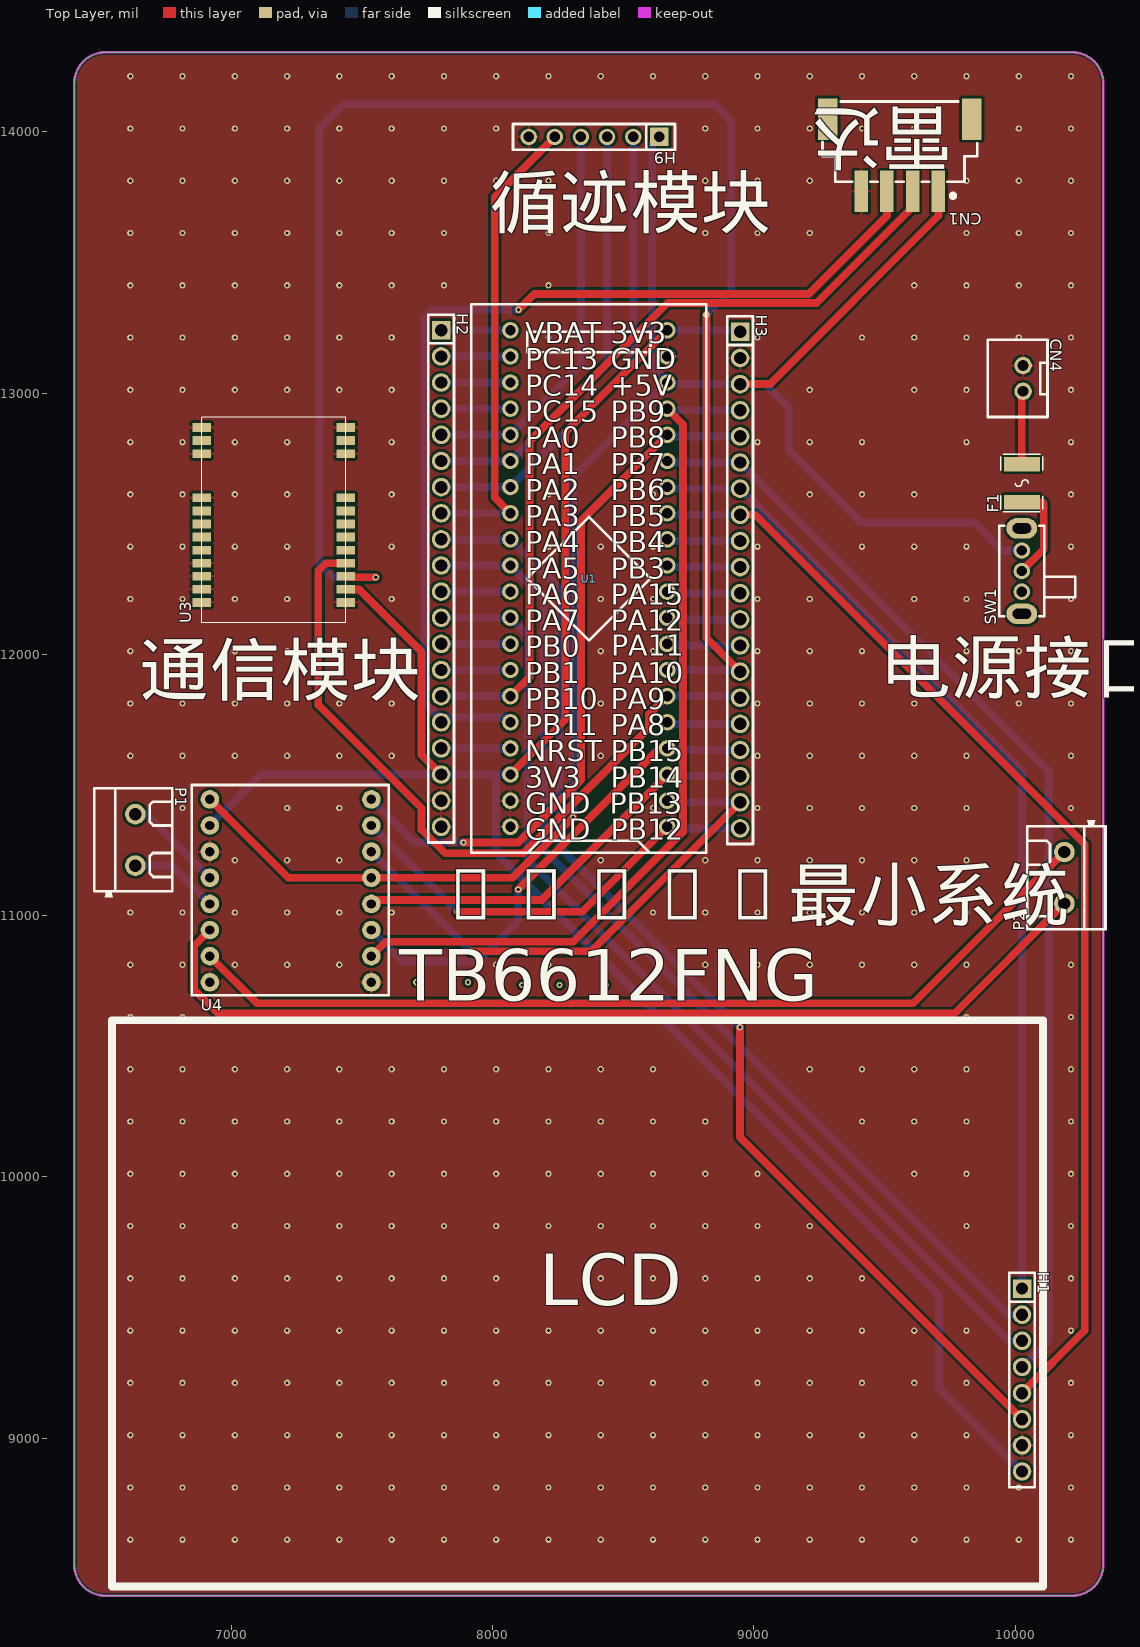
[diagram p0: Top Layer view]
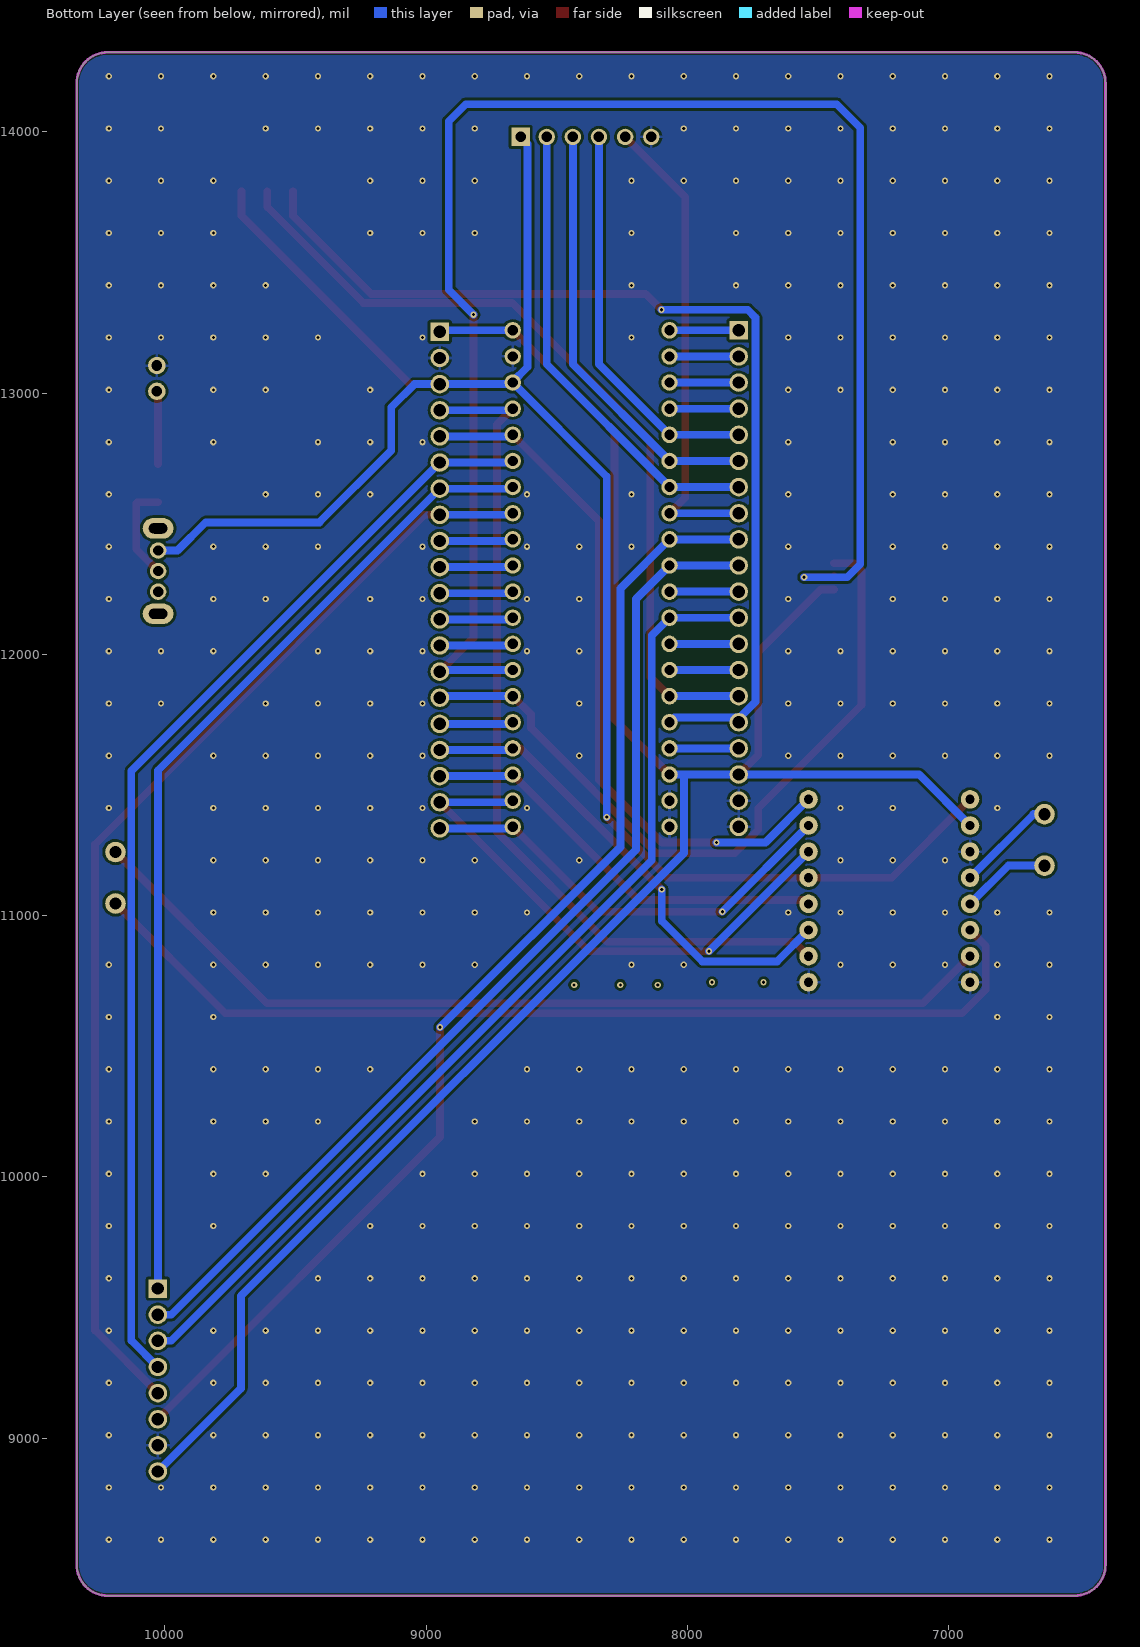
[diagram p1: Bottom Layer view, seen from below]
# Altium PCB MISC52128.pcbdoc
Units mil, origin at the board's own origin, x right, y up, seen from the top; angles counter-clockwise.
Board outline 3937.01 x 5905.51 mil, 2 copper layers (Top Layer, Bottom Layer), stack 62.206 mil thick; 13 components, 43 nets, 153 pads, 421 vias.

## Layer stack, top to bottom
Top Solder Mask Layer: solder mask 0.394, Dk 3.3
Top Layer: signal copper 1.379
Dielectric1: surface 59.449, FR4, Dk 4.5
Bottom Layer: signal copper 1.378
Bottom Solder Mask Layer: solder mask 0.394, Dk 3.3

## Board outline
6517.91,14303.5 ccw(c6517.91,14185.39) 6399.8,14185.39 6399.8,8516.1 ccw(c6517.91,8516.1) 6517.91,8397.99 10218.7,8397.99 ccw(c10218.7,8516.1) 10336.81,8516.1 10336.81,14185.39 ccw(c10218.7,14185.39) 10218.7,14303.5 6517.91,14303.5

## Design rules (kind name [scope] priority, off if disabled: settings)
BoardOutlineClearance copperThickness2oz_1 [All] p2 off: genericclearance=7.99 ignorepadtopadclearanceinfootprint=FALSE except(0: Arc-SplitContinuation Track-SplitContinuation SMDPad-SplitContinuation THPad-SplitContinuation Via-SplitContinuation Fill-SplitContinuation Region-SplitContinuation Poly-SplitContinuation Text-SplitContinuation Hole-SplitContinuation; 5.98: Arc-CutoutEdge Track-CutoutEdge SMDPad-CutoutEdge THPad-CutoutEdge Via-CutoutEdge Text-CutoutEdge; 6.9: Hole-OutlineEdge Hole-CutoutEdge; 10: Poly-OutlineEdge Poly-CutoutEdge; 11.81: Arc-OutlineEdge Track-OutlineEdge SMDPad-OutlineEdge THPad-OutlineEdge Via-OutlineEdge Fill-OutlineEdge Region-OutlineEdge Text-OutlineEdge Fill-CutoutEdge Region-CutoutEdge)
BoardOutlineClearance Plane_innerPlane_1 [All] p4 off: genericclearance=4.02 ignorepadtopadclearanceinfootprint=FALSE except(0: Arc-SplitContinuation Track-SplitContinuation SMDPad-SplitContinuation THPad-SplitContinuation Via-SplitContinuation Fill-SplitContinuation Region-SplitContinuation Poly-SplitContinuation Text-SplitContinuation Hole-SplitContinuation; 5.98: Arc-CutoutEdge Track-CutoutEdge SMDPad-CutoutEdge THPad-CutoutEdge Via-CutoutEdge Text-CutoutEdge; 6.9: Hole-OutlineEdge Hole-CutoutEdge; 10: Poly-OutlineEdge Poly-CutoutEdge; 11.81: Arc-OutlineEdge Track-OutlineEdge SMDPad-OutlineEdge THPad-OutlineEdge Via-OutlineEdge Fill-OutlineEdge Region-OutlineEdge Text-OutlineEdge Fill-CutoutEdge Region-CutoutEdge)
BoardOutlineClearance Copper_copperRegion_1 [All] p6 off: genericclearance=4.02 ignorepadtopadclearanceinfootprint=FALSE except(0: Arc-SplitContinuation Track-SplitContinuation SMDPad-SplitContinuation THPad-SplitContinuation Via-SplitContinuation Fill-SplitContinuation Region-SplitContinuation Poly-SplitContinuation Text-SplitContinuation Hole-SplitContinuation; 5.98: Arc-CutoutEdge Track-CutoutEdge SMDPad-CutoutEdge THPad-CutoutEdge Via-CutoutEdge Text-CutoutEdge; 6.9: Hole-OutlineEdge Hole-CutoutEdge; 10: Poly-OutlineEdge Poly-CutoutEdge; 11.81: Arc-OutlineEdge Track-OutlineEdge SMDPad-OutlineEdge THPad-OutlineEdge Via-OutlineEdge Fill-OutlineEdge Region-OutlineEdge Text-OutlineEdge Fill-CutoutEdge Region-CutoutEdge)
BoardOutlineClearance Copper_copperRegion_copperThickness1oz_1 [All] p8 off: genericclearance=4.02 ignorepadtopadclearanceinfootprint=FALSE except(0: Arc-SplitContinuation Track-SplitContinuation SMDPad-SplitContinuation THPad-SplitContinuation Via-SplitContinuation Fill-SplitContinuation Region-SplitContinuation Poly-SplitContinuation Text-SplitContinuation Hole-SplitContinuation; 5.98: Arc-CutoutEdge Track-CutoutEdge SMDPad-CutoutEdge THPad-CutoutEdge Via-CutoutEdge Text-CutoutEdge; 6.9: Hole-OutlineEdge Hole-CutoutEdge; 10: Poly-OutlineEdge Poly-CutoutEdge; 11.81: Arc-OutlineEdge Track-OutlineEdge SMDPad-OutlineEdge THPad-OutlineEdge Via-OutlineEdge Fill-OutlineEdge Region-OutlineEdge Text-OutlineEdge Fill-CutoutEdge Region-CutoutEdge)
BoardOutlineClearance Copper_copperRegion_Copper_copperRegion_1 [All] p10 off: genericclearance=4.02 ignorepadtopadclearanceinfootprint=FALSE except(0: Arc-SplitContinuation Track-SplitContinuation SMDPad-SplitContinuation THPad-SplitContinuation Via-SplitContinuation Fill-SplitContinuation Region-SplitContinuation Poly-SplitContinuation Text-SplitContinuation Hole-SplitContinuation; 5.98: Arc-CutoutEdge Track-CutoutEdge SMDPad-CutoutEdge THPad-CutoutEdge Via-CutoutEdge Text-CutoutEdge; 6.9: Hole-OutlineEdge Hole-CutoutEdge; 10: Poly-OutlineEdge Poly-CutoutEdge; 11.81: Arc-OutlineEdge Track-OutlineEdge SMDPad-OutlineEdge THPad-OutlineEdge Via-OutlineEdge Fill-OutlineEdge Region-OutlineEdge Text-OutlineEdge Fill-CutoutEdge Region-CutoutEdge)
BoardOutlineClearance copperThickness1oz_1 [All] p12: genericclearance=4.02 ignorepadtopadclearanceinfootprint=FALSE except(0: Arc-SplitContinuation Track-SplitContinuation SMDPad-SplitContinuation THPad-SplitContinuation Via-SplitContinuation Fill-SplitContinuation Region-SplitContinuation Poly-SplitContinuation Text-SplitContinuation Hole-SplitContinuation; 5.98: Arc-CutoutEdge Track-CutoutEdge SMDPad-CutoutEdge THPad-CutoutEdge Via-CutoutEdge Text-CutoutEdge; 6.9: Hole-OutlineEdge Hole-CutoutEdge; 10: Poly-OutlineEdge Poly-CutoutEdge; 11.81: Arc-OutlineEdge Track-OutlineEdge SMDPad-OutlineEdge THPad-OutlineEdge Via-OutlineEdge Fill-OutlineEdge Region-OutlineEdge Text-OutlineEdge Fill-CutoutEdge Region-CutoutEdge)
Clearance copperThickness2oz [All] p1 off: gap=7.99 ignorepadtopadclearanceinfootprint=FALSE except(5.98: SMDPad-Track SMDPad-SMDPad THPad-Track SMDPad-THPad THPad-THPad Track-Via SMDPad-Via THPad-Via Via-Via Fill-SMDPad Region-SMDPad Fill-THPad Region-THPad Fill-Via Region-Via Fill-Fill Fill-Region Region-Region Arc-Track Arc-SMDPad Arc-THPad Arc-Via Fill-Arc Region-Arc Arc-Arc Text-Track SMDPad-Text Text-THPad Text-Via Fill-Text Region-Text Arc-Text Text-Text; 6.9: Hole-Track Hole-SMDPad Hole-THPad Hole-Via Fill-Hole Region-Hole Hole-Arc Hole-Text; 10: Poly-Track Poly-SMDPad Poly-THPad Poly-Via Poly-Fill Poly-Region Poly-Poly Poly-Arc Poly-Text Poly-Hole; 11.81: Fill-Track Region-Track)
Clearance Plane_innerPlane [All] p3 off: gap=4.02 ignorepadtopadclearanceinfootprint=FALSE except(5.98: SMDPad-Track SMDPad-SMDPad THPad-Track SMDPad-THPad THPad-THPad Track-Via SMDPad-Via THPad-Via Via-Via Fill-SMDPad Region-SMDPad Fill-THPad Region-THPad Fill-Via Region-Via Fill-Fill Fill-Region Region-Region Arc-Track Arc-SMDPad Arc-THPad Arc-Via Fill-Arc Region-Arc Arc-Arc Text-Track SMDPad-Text Text-THPad Text-Via Fill-Text Region-Text Arc-Text Text-Text; 6.9: Hole-Track Hole-SMDPad Hole-THPad Hole-Via Fill-Hole Region-Hole Hole-Arc Hole-Text; 10: Poly-Track Poly-SMDPad Poly-THPad Poly-Via Poly-Fill Poly-Region Poly-Poly Poly-Arc Poly-Text Poly-Hole; 11.81: Fill-Track Region-Track)
Clearance Copper_copperRegion [All] p5 off: gap=4.02 ignorepadtopadclearanceinfootprint=FALSE except(5.98: SMDPad-Track SMDPad-SMDPad THPad-Track SMDPad-THPad THPad-THPad Track-Via SMDPad-Via THPad-Via Via-Via Fill-SMDPad Region-SMDPad Fill-THPad Region-THPad Fill-Via Region-Via Fill-Fill Fill-Region Region-Region Arc-Track Arc-SMDPad Arc-THPad Arc-Via Fill-Arc Region-Arc Arc-Arc Text-Track SMDPad-Text Text-THPad Text-Via Fill-Text Region-Text Arc-Text Text-Text; 6.9: Hole-Track Hole-SMDPad Hole-THPad Hole-Via Fill-Hole Region-Hole Hole-Arc Hole-Text; 10: Poly-Track Poly-SMDPad Poly-THPad Poly-Via Poly-Fill Poly-Region Poly-Poly Poly-Arc Poly-Text Poly-Hole; 11.81: Fill-Track Region-Track)
Clearance Copper_copperRegion_copperThickness1oz [All] p7 off: gap=4.02 ignorepadtopadclearanceinfootprint=FALSE except(5.98: SMDPad-Track SMDPad-SMDPad THPad-Track SMDPad-THPad THPad-THPad Track-Via SMDPad-Via THPad-Via Via-Via Fill-SMDPad Region-SMDPad Fill-THPad Region-THPad Fill-Via Region-Via Fill-Fill Fill-Region Region-Region Arc-Track Arc-SMDPad Arc-THPad Arc-Via Fill-Arc Region-Arc Arc-Arc Text-Track SMDPad-Text Text-THPad Text-Via Fill-Text Region-Text Arc-Text Text-Text; 6.9: Hole-Track Hole-SMDPad Hole-THPad Hole-Via Fill-Hole Region-Hole Hole-Arc Hole-Text; 10: Poly-Track Poly-SMDPad Poly-THPad Poly-Via Poly-Fill Poly-Region Poly-Poly Poly-Arc Poly-Text Poly-Hole; 11.81: Fill-Track Region-Track)
Clearance Copper_copperRegion_Copper_copperRegion [All] p9 off: gap=4.02 ignorepadtopadclearanceinfootprint=FALSE except(5.98: SMDPad-Track SMDPad-SMDPad THPad-Track SMDPad-THPad THPad-THPad Track-Via SMDPad-Via THPad-Via Via-Via Fill-SMDPad Region-SMDPad Fill-THPad Region-THPad Fill-Via Region-Via Fill-Fill Fill-Region Region-Region Arc-Track Arc-SMDPad Arc-THPad Arc-Via Fill-Arc Region-Arc Arc-Arc Text-Track SMDPad-Text Text-THPad Text-Via Fill-Text Region-Text Arc-Text Text-Text; 6.9: Hole-Track Hole-SMDPad Hole-THPad Hole-Via Fill-Hole Region-Hole Hole-Arc Hole-Text; 10: Poly-Track Poly-SMDPad Poly-THPad Poly-Via Poly-Fill Poly-Region Poly-Poly Poly-Arc Poly-Text Poly-Hole; 11.81: Fill-Track Region-Track)
Clearance copperThickness1oz [All] p11: gap=4.02 ignorepadtopadclearanceinfootprint=FALSE except(5.98: SMDPad-Track SMDPad-SMDPad THPad-Track SMDPad-THPad THPad-THPad Track-Via SMDPad-Via THPad-Via Via-Via Fill-SMDPad Region-SMDPad Fill-THPad Region-THPad Fill-Via Region-Via Fill-Fill Fill-Region Region-Region Arc-Track Arc-SMDPad Arc-THPad Arc-Via Fill-Arc Region-Arc Arc-Arc Text-Track SMDPad-Text Text-THPad Text-Via Fill-Text Region-Text Arc-Text Text-Text; 6.9: Hole-Track Hole-SMDPad Hole-THPad Hole-Via Fill-Hole Region-Hole Hole-Arc Hole-Text; 10: Poly-Track Poly-SMDPad Poly-THPad Poly-Via Poly-Fill Poly-Region Poly-Poly Poly-Arc Poly-Text Poly-Hole; 11.81: Fill-Track Region-Track)
DiffPairsRouting differentialPair [All] p1: maxlimit=6 minlimit=6 mostfreqgap=6 toplayer_minwidth=5 toplayer_prefwidth=10 toplayer_maxwidth=100 toplayer_mingap=6 toplayer_prefgap=6 toplayer_maxgap=6 bottomlayer_minwidth=5 bottomlayer_prefwidth=10 bottomlayer_maxwidth=100 bottomlayer_mingap=6 bottomlayer_prefgap=6 bottomlayer_maxgap=6 maxuncoupledlength=10
HoleToHoleClearance otherClearance [All] p1: gap=11.81 allowstackedmicrovias=TRUE
Length netLength [All] p1: minlimit=0 maxlimit=0
MatchedLengths netLengthTolerance [All] p1: tolerance=1000
PasteMaskExpansion pasteMaskExpansion [All] p1: expansion=0
PlaneConnect innerPlane [All] p1: planeconnectstyle=Relief reliefexpansion=20 reliefentries=4 reliefconductorwidth=10 reliefairgap=10
PolygonConnect copperRegion_copperThickness1oz [All] p1 off: connectstyle=Relief reliefconductorwidth=10 reliefentries=4 polygonreliefangle="90 Angle" airgapwidth=10 via.connectstyle=Relief via.reliefconductorwidth=10 via.reliefentries=4 via.polygonreliefangle="90 Angle" via.airgapwidth=10
PolygonConnect copperRegion_Copper_copperRegion [All] p2 off: connectstyle=Relief reliefconductorwidth=10 reliefentries=4 polygonreliefangle="90 Angle" airgapwidth=10 via.connectstyle=Relief via.reliefconductorwidth=10 via.reliefentries=4 via.polygonreliefangle="90 Angle" via.airgapwidth=10
PolygonConnect copperRegion [All] p3: connectstyle=Relief reliefconductorwidth=10 reliefentries=4 polygonreliefangle="90 Angle" airgapwidth=10 via.connectstyle=Relief via.reliefconductorwidth=10 via.reliefentries=4 via.polygonreliefangle="90 Angle" via.airgapwidth=10
RoutingVias viaSize [All] p1: holewidth=12.01 width=24.02 viastyle="Through Hole" minholewidth=11.81 minwidth=19.68 maxholewidth=248.03 maxwidth=393.7
SolderMaskExpansion solderMaskExpansion [IsVia] p1: expansion=-1000 istentingtop=TRUE
SolderMaskExpansion solderMaskExpansion [All] p2: expansion=2 istentingtop=FALSE
Width copperThickness2oz_2 [All] p1 off: maxlimit=100 minlimit=8 preferedwidth=10
Width copperThickness1oz_2 [All] p2: maxlimit=10 minlimit=10 preferedwidth=10 toplayer_minwidth=30 toplayer_maxwidth=100 toplayer_prefwidth=30 bottomlayer_minwidth=30 bottomlayer_maxwidth=100 bottomlayer_prefwidth=30

## Components (designator, comment, footprint, x,y, rotation, side; value= is the part's Value field where it differs from the comment)
CN1 "XH2.54-4P" CONN-SMD_4P-P2.50-WT 9558.31,13910 r180 top
CN4 "XH2.54*2P_直插" CONN-TH_2P-P2.50-XH2.54-2P 10030.3,13055.81 r270 top
F1 "SMD1812-300-24" F1812 10025.33,12655.04 r90 top
H1 "" HDR-TH_8P-P2.54-V-F-1 10026.3,9223.07 r270 top
H2 "" HDR-TH_20P-P2.54-V-F 7803.31,12290 r270 top
H3 "" HDR-TH_20P-P2.54-V-F 8947.41,12283.94 r270 top
H9 "" HDR-TH_6P-P2.54-V-F 8388.31,13980 r180 top
P1 "KF301-2P接线端子" CONN-TH_XY301V-A-5.0-2P 6633.31,11290 r270 top
P2 "KF301-2P接线端子" CONN-TH_XY301V-A-5.0-2P 10188.31,11145 r90 top
SW1 "" 拨动开关_侧 10025.33,12318.57 r90 top
U1 "STM32F103C8T6-Card" CONN-TH_L53.3-W22.9_STM32F103C8T6-CARD 8368.31,12290 r90 top
U3 "" EWM22M-400/900T22S 7438.31,12120 r90 top
U4 "" tb6612 6918.31,11445 r0 top

## Footprints (in the part's own frame and the unit in brackets; to place one, negate y for a bottom-side part, rotate by r counter-clockwise, add the part's x,y. Pads: shape width x height; smd on the part's side, far side on the other; paste and mask are expansions set on the pad)
CONN-SMD_4P-P2.50-WT [mm]
  rect 1.3x4 smd: 1(-3.75,3.5) 2(-1.25,3.5) 3(1.25,3.5) 4(3.75,3.5)
  rect 1.9x4 smd: 5(7,-3.5) 6(-7,-3.5)
  silkscreen extent -7.53,-5.22 7.51,4.14
CONN-TH_2P-P2.50-XH2.54-2P [mm]
  round 1.7 hole 1.05 paste+0 mask+0.05: 1(1.25,0) 2(-1.25,0)
  silkscreen extent -3.75,-3.42 3.75,2.37
CONN-TH_L53.3-W22.9_STM32F103C8T6-CARD [mm]
  round 1.6 hole 1: 1(-24.13,-7.62) 2(-21.59,-7.62) 3(-19.05,-7.62) 4(-16.51,-7.62) 5(-13.97,-7.62) 6(-11.43,-7.62) 7(-8.89,-7.62) 8(-6.35,-7.62) 9(-3.81,-7.62) 10(-1.27,-7.62) 11(1.27,-7.62) 12(3.81,-7.62) 13(6.35,-7.62) 14(8.89,-7.62) 15(11.43,-7.62) 16(13.97,-7.62) 17(16.51,-7.62) 18(19.05,-7.62) 19(21.59,-7.62) 20(24.13,-7.62) 21(24.13,7.62) 22(21.59,7.62) 23(19.05,7.62) 24(16.51,7.62) 25(13.97,7.62) 26(11.43,7.62) 27(8.89,7.62) 28(6.35,7.62) 29(3.81,7.62) 30(1.27,7.62) 31(-1.27,7.62) 32(-3.81,7.62) 33(-6.35,7.62) 34(-8.89,7.62) 35(-11.43,7.62) 36(-13.97,7.62) 37(-16.51,7.62) 38(-19.05,7.62) 39(-21.59,7.62) 40(-24.13,7.62)
  silkscreen extent -26.67,-11.43 26.67,11.43
CONN-TH_XY301V-A-5.0-2P [mm]
  round 2 hole 1.2: 1(-2.5,0) 2(2.5,0)
  silkscreen extent -5,-4 5.6,3.6
EWM22M-400/900T22S [mm]
  rect 0.85x1.8 smd: 1(19,14) 2(17.73,14) 3(16.46,14) 4(12.16,14) 5(10.89,14) 6(9.62,14) 7(8.35,14) 8(7.08,14) 9(5.81,14) 10(4.54,14) 11(3.27,14) 12(2,14) 13(2,0) 14(3.27,0) 15(4.54,0) 16(5.81,0) 17(7.08,0) 18(8.35,0) 19(9.62,0) 20(10.89,0) 21(12.16,0) 22(16.46,0) 23(17.73,0) 24(19,0)
  silkscreen extent 0,0 20,14
F1812 [mil]
  rect 55.38x137.76 smd paste-3937.01 mask+2: 1(-72.97,0) 2(72.97,0)
  silkscreen extent -110,-80 110,80
HDR-TH_6P-P2.54-V-F [mm]
  rect 1.8x1.8 hole 1.02: 1(-6.35,0)
  round 1.6 hole 1.02: 2(-3.81,0) 3(-1.27,0) 4(1.27,0) 5(3.81,0) 6(6.35,0)
  silkscreen extent -7.87,-1.25 7.87,1.25
HDR-TH_8P-P2.54-V-F-1 [mm]
  rect 1.8x1.8 hole 1.2: 1(-8.89,0)
  round 1.8 hole 1.2: 2(-6.35,0) 3(-3.81,0) 4(-1.27,0) 5(1.27,0) 6(3.81,0) 7(6.35,0) 8(8.89,0)
  silkscreen extent -10.41,-1.25 10.41,1.25
HDR-TH_20P-P2.54-V-F [mm]
  rect 1.8x1.8 hole 1.2: 1(-24.13,0)
  round 1.8 hole 1.2: 2(-21.59,0) 3(-19.05,0) 4(-16.51,0) 5(-13.97,0) 6(-11.43,0) 7(-8.89,0) 8(-6.35,0) 9(-3.81,0) 10(-1.27,0) 11(1.27,0) 12(3.81,0) 13(6.35,0) 14(8.89,0) 15(11.43,0) 16(13.97,0) 17(16.51,0) 18(19.05,0) 19(21.59,0) 20(24.13,0)
  silkscreen extent -25.65,-1.25 25.65,1.25
tb6612 [mm]
  round 1.8 hole 0.9: 1(0,0) 2(0,-2.54) 3(0,-5.08) 4(0,-7.62) 5(0,-10.16) 6(0,-12.7) 7(0,-15.24) 8(0,-17.78) 9(15.697,-17.78) 10(15.697,-15.24) 11(15.697,-12.7) 12(15.697,-10.16) 13(15.697,-7.62) 14(15.697,-5.08) 15(15.697,-2.54) 16(15.697,0)
  silkscreen extent -1.78,-19.05 17.4,1.4
拨动开关_侧 [mil]
  round 63 hole 39.4 paste+0 mask+2: 1(-78.7,0) 2(0,0) 3(78.7,0)
  oval 78.7x118.1 hole 39.4 slot 70.9 at 90 deg paste+0 mask+2: 4(163.4,0) 5(-163.4,0)
  silkscreen extent -173,-205 173,87

## Via types
v1: diameter 24.02, hole 12, Top Layer to Bottom Layer, 421 vias

## Nets (pads, with @x,y where several pads share a name; then routed paths per layer and width w, separated by ;. In a path a pad name is that pad's centre, name@x,y a point inside that pad or via, vN(x,y) a via of type N, cw(c..) or ccw(c..) an arc to the next point about the centre after c; other vN are vias at no path point)
$1N17273: P1.1 U4.4 | length 385.8
  Bottom Layer w30: P1.1 6674.88,11388.42 U4.4
$1N17274: P1.2 U4.5 | length 345.7
  Bottom Layer w30: P1.2 6771.73,11191.57 U4.5
$1N17275: P2.1 U4.6 | length 3794.5
  Top Layer w30: U4.6 6858.31,10885 6858.31,10716.58 6948.31,10626.58 9768.31,10626.58 P2.1
$1N17276: P2.2 U4.7 | length 3584.1
  Top Layer w30: U4.7 7098.31,10665 9609.88,10665 P2.2
$1N17293: CN4.1 F1.2 | length 280.6
  Top Layer w30: F1.2 10025.33,13001.63 CN4.1
$1N17294: F1.1 SW1.2 | length 379.1
  Top Layer w30: SW1.2 10109.22,12402.45 10109.22,12576.93 10104.07,12582.07 F1.1
+5V: CN1.1 H3.3 H9.1 SW1.3 U1.18 U4.1 U4.13 | length 7237.7
  Top Layer w30: U4.1 7218.31,11145 U4.13 8076.31,11145 v1(8308.31,11377) ; H3.3 9061.42,13033.94 9705.95,13678.46 CN1.1
  Bottom Layer w30: v1(8308.31,11377) 8308.31,12680 U1.18 U1.18@8671.35,13040 ; H9.1 8611.35,13953.04 8611.35,13100 U1.18@8671.35,13040 ; SW1.3 9951.04,12397.27 9843.31,12505 9408.31,12505 9133.31,12780 9133.31,12945 9044.37,13033.94 H3.3 8677.42,13033.94 U1.18@8671.35,13040
GND: CN1.4 CN4.2 H1.7 H2.19 H2.20 H3.2 H9.6 U1.19 U1.39 U1.40 U3.1 U3.3 U3.4 U3.9 U3.10 U3.11 U3.12 U3.13 U3.22 U3.24 U4.3 U4.8 U4.9
  other v1: 6613.9,8612.09 6813.9,8612.09 7013.9,8612.09 7213.9,8612.09 7413.9,8612.09 7613.9,8612.09 7813.9,8612.09 8013.9,8612.09 8213.9,8612.09 8413.9,8612.09 8613.9,8612.09 8813.9,8612.09 9013.9,8612.09 9213.9,8612.09 9413.9,8612.09 9613.9,8612.09 9813.9,8612.09 10013.9,8612.09 10213.9,8612.09 6613.9,8812.09 6813.9,8812.09 7013.9,8812.09 7213.9,8812.09 7413.9,8812.09 7613.9,8812.09 7813.9,8812.09 8013.9,8812.09 8213.9,8812.09 8413.9,8812.09 8613.9,8812.09 8813.9,8812.09 9013.9,8812.09 9213.9,8812.09 9413.9,8812.09 9613.9,8812.09 9813.9,8812.09 10013.9,8812.09 10213.9,8812.09 6613.9,9012.09 6813.9,9012.09 7013.9,9012.09 7213.9,9012.09 7413.9,9012.09 7613.9,9012.09 7813.9,9012.09 8013.9,9012.09 8213.9,9012.09 8413.9,9012.09 8613.9,9012.09 8813.9,9012.09 9013.9,9012.09 9213.9,9012.09 9413.9,9012.09 9613.9,9012.09 9813.9,9012.09 10213.9,9012.09 6613.9,9212.09 6813.9,9212.09 7013.9,9212.09 7213.9,9212.09 7413.9,9212.09 7613.9,9212.09 7813.9,9212.09 8013.9,9212.09 8213.9,9212.09 8413.9,9212.09 8613.9,9212.09 8813.9,9212.09 9013.9,9212.09 9213.9,9212.09 9413.9,9212.09 9613.9,9212.09 9813.9,9212.09 10213.9,9212.09 6613.9,9412.09 6813.9,9412.09 7013.9,9412.09 7213.9,9412.09 7413.9,9412.09 7613.9,9412.09 7813.9,9412.09 8013.9,9412.09 8213.9,9412.09 8413.9,9412.09 8613.9,9412.09 8813.9,9412.09 9013.9,9412.09 9213.9,9412.09 9413.9,9412.09 9613.9,9412.09 9813.9,9412.09 10213.9,9412.09 6613.9,9612.09 6813.9,9612.09 7013.9,9612.09 7213.9,9612.09 7413.9,9612.09 7613.9,9612.09 7813.9,9612.09 8013.9,9612.09 8213.9,9612.09 8413.9,9612.09 8613.9,9612.09 8813.9,9612.09 9013.9,9612.09 9213.9,9612.09 9413.9,9612.09 10213.9,9612.09 6613.9,9812.09 6813.9,9812.09 7013.9,9812.09 7213.9,9812.09 7413.9,9812.09 7613.9,9812.09 7813.9,9812.09 8013.9,9812.09 8213.9,9812.09 8413.9,9812.09 8613.9,9812.09 8813.9,9812.09 9013.9,9812.09 9213.9,9812.09 9813.9,9812.09 10213.9,9812.09 6613.9,10012.09 6813.9,10012.09 7013.9,10012.09 7213.9,10012.09 7413.9,10012.09 7613.9,10012.09 7813.9,10012.09 8013.9,10012.09 8213.9,10012.09 8413.9,10012.09 8613.9,10012.09 8813.9,10012.09 9013.9,10012.09 9613.9,10012.09 9813.9,10012.09 10213.9,10012.09 6613.9,10212.09 6813.9,10212.09 7013.9,10212.09 7213.9,10212.09 7413.9,10212.09 7613.9,10212.09 7813.9,10212.09 8013.9,10212.09 8213.9,10212.09 8413.9,10212.09 8613.9,10212.09 8813.9,10212.09 9413.9,10212.09 9613.9,10212.09 9813.9,10212.09 10213.9,10212.09 6613.9,10412.09 6813.9,10412.09 7013.9,10412.09 7213.9,10412.09 7413.9,10412.09 7613.9,10412.09 7813.9,10412.09 8013.9,10412.09 8213.9,10412.09 8413.9,10412.09 8613.9,10412.09 9213.9,10412.09 9413.9,10412.09 9613.9,10412.09 9813.9,10412.09 10213.9,10412.09 6613.9,10612.09 6813.9,10612.09 9813.9,10612.09 10213.9,10612.09 6613.9,10812.09 6813.9,10812.09 7013.9,10812.09 7213.9,10812.09 7413.9,10812.09 8013.9,10812.09 8213.9,10812.09 8813.9,10812.09 9013.9,10812.09 9213.9,10812.09 9413.9,10812.09 9613.9,10812.09 9813.9,10812.09 10213.9,10812.09 6613.9,11012.09 6813.9,11012.09 7013.9,11012.09 7213.9,11012.09 7413.9,11012.09 7613.9,11012.09 8613.9,11012.09 8813.9,11012.09 9013.9,11012.09 9213.9,11012.09 9413.9,11012.09 9613.9,11012.09 9813.9,11012.09 7013.9,11212.09 7213.9,11212.09 7413.9,11212.09 8413.9,11212.09 8813.9,11212.09 9013.9,11212.09 9213.9,11212.09 9413.9,11212.09 9613.9,11212.09 9813.9,11212.09 6813.9,11412.09 7213.9,11412.09 7413.9,11412.09 8613.9,11412.09 9013.9,11412.09 9213.9,11412.09 9413.9,11412.09 9613.9,11412.09 9813.9,11412.09 10213.9,11412.09 6613.9,11612.09 6813.9,11612.09 7013.9,11612.09 7213.9,11612.09 7413.9,11612.09 7613.9,11612.09 8413.9,11612.09 9013.9,11612.09 9213.9,11612.09 9413.9,11612.09 9613.9,11612.09 9813.9,11612.09 10213.9,11612.09 6613.9,11812.09 6813.9,11812.09 7013.9,11812.09 7213.9,11812.09 7413.9,11812.09 7613.9,11812.09 8413.9,11812.09 9013.9,11812.09 9213.9,11812.09 9413.9,11812.09 9613.9,11812.09 10013.9,11812.09 10213.9,11812.09 6613.9,12012.09 6813.9,12012.09 7013.9,12012.09 7213.9,12012.09 7413.9,12012.09 7613.9,12012.09 8413.9,12012.09 8613.9,12012.09 9013.9,12012.09 9213.9,12012.09 9413.9,12012.09 9813.9,12012.09 10013.9,12012.09 10213.9,12012.09 6613.9,12212.09 6813.9,12212.09 7013.9,12212.09 7213.9,12212.09 7613.9,12212.09 8413.9,12212.09 8613.9,12212.09 9013.9,12212.09 9213.9,12212.09 9613.9,12212.09 9813.9,12212.09 10213.9,12212.09 6613.9,12412.09 6813.9,12412.09 7013.9,12412.09 7213.9,12412.09 7613.9,12412.09 8213.9,12412.09 8413.9,12412.09 8613.9,12412.09 9013.9,12412.09 9413.9,12412.09 9613.9,12412.09 9813.9,12412.09 10213.9,12412.09 6613.9,12612.09 6813.9,12612.09 7013.9,12612.09 7213.9,12612.09 7613.9,12612.09 8213.9,12612.09 8613.9,12612.09 9213.9,12612.09 9413.9,12612.09 9613.9,12612.09 10213.9,12612.09 6613.9,12812.09 6813.9,12812.09 7013.9,12812.09 7213.9,12812.09 7613.9,12812.09 9013.9,12812.09 9213.9,12812.09 9413.9,12812.09 9813.9,12812.09 10213.9,12812.09 6613.9,13012.09 6813.9,13012.09 7013.9,13012.09 7213.9,13012.09 7413.9,13012.09 7613.9,13012.09 9213.9,13012.09 9613.9,13012.09 9813.9,13012.09 10213.9,13012.09 6613.9,13212.09 6813.9,13212.09 7013.9,13212.09 7213.9,13212.09 7413.9,13212.09 7613.9,13212.09 8213.9,13212.09 9013.9,13212.09 9413.9,13212.09 9613.9,13212.09 9813.9,13212.09 10013.9,13212.09 10213.9,13212.09 6613.9,13412.09 6813.9,13412.09 7013.9,13412.09 7213.9,13412.09 7413.9,13412.09 7613.9,13412.09 7813.9,13412.09 8213.9,13412.09 9613.9,13412.09 9813.9,13412.09 10013.9,13412.09 10213.9,13412.09 6613.9,13612.09 6813.9,13612.09 7013.9,13612.09 7213.9,13612.09 7413.9,13612.09 7613.9,13612.09 7813.9,13612.09 8213.9,13612.09 8813.9,13612.09 9013.9,13612.09 9213.9,13612.09 9813.9,13612.09 10013.9,13612.09 10213.9,13612.09 6613.9,13812.09 6813.9,13812.09 7013.9,13812.09 7213.9,13812.09 7413.9,13812.09 7613.9,13812.09 7813.9,13812.09 8013.9,13812.09 8213.9,13812.09 8813.9,13812.09 9013.9,13812.09 9213.9,13812.09 9813.9,13812.09 10013.9,13812.09 10213.9,13812.09 6613.9,14012.09 6813.9,14012.09 7013.9,14012.09 7213.9,14012.09 7413.9,14012.09 7613.9,14012.09 7813.9,14012.09 8013.9,14012.09 8813.9,14012.09 9013.9,14012.09 9213.9,14012.09 9413.9,14012.09 9613.9,14012.09 10013.9,14012.09 10213.9,14012.09 6613.9,14212.09 6813.9,14212.09 7013.9,14212.09 7213.9,14212.09 7413.9,14212.09 7613.9,14212.09 7813.9,14212.09 8013.9,14212.09 8213.9,14212.09 8413.9,14212.09 8613.9,14212.09 8813.9,14212.09 9013.9,14212.09 9213.9,14212.09 9413.9,14212.09 9613.9,14212.09 9813.9,14212.09 10013.9,14212.09 10213.9,14212.09
NRST: H2.17 U1.37 | length 265
  Bottom Layer w30: H2.17 U1.37
PA0: H2.5 H9.4 U1.25 | length 1516.8
  Bottom Layer w30: H2.5 U1.25 8338.31,13110 H9.4
PA1: H2.6 H9.3 U1.26 | length 1658.2
  Bottom Layer w30: H2.6 U1.26 8438.31,13110 H9.3
PA2: H2.7 H9.2 U1.27 | length 1799.7
  Bottom Layer w30: H2.7 U1.27 8538.31,13110 H9.2
PA3: H2.8 H9.5 U1.28 | length 1825.1
  Top Layer w30: U1.28 8008.31,12600 8008.31,13750 H9.5
  Bottom Layer w30: H2.8 U1.28
PA4: H1.6 H2.9 U1.29 | length 4443
  Top Layer w30: v1(8946.3,10573.07) 8946.3,10153.07 H1.6
  Bottom Layer w30: H2.9 U1.29 8256.3,12252.01 8256.3,11263.07 v1(8946.3,10573.07)
PA5: H1.2 H2.10 U1.30 | length 3972.9
  Bottom Layer w30: H2.10 U1.30 8196.3,12212.01 8196.3,11252.01 9975.24,9473.07 H1.2
PA6: H2.11 U1.31 | length 265
  Bottom Layer w30: H2.11 U1.31
PA7: H1.3 H2.12 U1.32 | length 3872.9
  Bottom Layer w30: H2.12 U1.32 8136.3,12072.01 8136.3,11212 9975.24,9373.07 H1.3
PA8: H3.16 U1.5 | length 281.6
  Bottom Layer w30: U1.5 8674.37,11733.94 H3.16
PA9: H3.15 U1.6 U3.16 | length 2809.8
  Top Layer w30: U3.16 7362.05,12348.74 7333.31,12320 7333.31,11806.7 7728.74,11411.26 7728.74,11328.74 7818.74,11238.74 8118.74,11238.74 8598.74,11718.74 8598.74,11770.44 U1.6
  Bottom Layer w30: U1.6 8941.35,11840 H3.15
PA10: H3.14 U1.7 U3.15 | length 6142
  Top Layer w30: U3.15 7442.05,12295 v1(7553.31,12295) ; v1(8818.31,13300) 8818.31,12063.04 H3.14
  Bottom Layer w30: v1(7553.31,12295) 7388.31,12295 7338.31,12345 7338.31,14015 7428.31,14105 8848.31,14105 8913.31,14040 8913.31,13395 v1(8818.31,13300) ; U1.7 8941.35,11940 H3.14
PA11: H3.13 U1.8 | length 281.6
  Bottom Layer w30: U1.8 8674.37,12033.94 H3.13
PA12: H3.12 U1.9 | length 281.6
  Bottom Layer w30: U1.9 8674.37,12133.94 H3.12
PA15: H3.11 U1.10 | length 281.6
  Bottom Layer w30: U1.10 8674.37,12233.94 H3.11
PB0: H2.13 U1.33 | length 265
  Bottom Layer w30: H2.13 U1.33
PB1: H2.14 U1.34 | length 265
  Bottom Layer w30: H2.14 U1.34
PB3: H3.10 U1.11 | length 281.6
  Bottom Layer w30: U1.11 8674.37,12333.94 H3.10
PB4: H3.9 U1.12 | length 281.6
  Bottom Layer w30: U1.12 8674.37,12433.94 H3.9
PB5: H1.5 H3.8 U1.13 | length 4322.2
  Top Layer w30: H3.8 9005.43,12533.94 10266.3,11273.07 10266.3,9413.07 H1.5
  Bottom Layer w30: U1.13 8674.37,12533.94 H3.8
PB6: H1.1 H3.7 U1.14 | length 3789.4
  Bottom Layer w30: U1.14 8674.37,12633.94 H3.7 10026.3,11555.05 H1.1
PB7: H1.4 H3.6 U1.15 | length 4273.6
  Bottom Layer w30: U1.15 8674.37,12733.94 H3.6 10127.95,11553.4 10127.95,9374.73 H1.4
PB8: H3.5 U1.16 U4.16 | length 2708.1
  Top Layer w30: v1(7888.31,11280.01) 8098.31,11280.01 8338.31,11520.01 8338.31,12510 U1.16
  Bottom Layer w30: U4.16 7701.3,11280.01 v1(7888.31,11280.01) ; U1.16 8674.37,12833.94 H3.5
PB9: H3.4 U1.17 U4.10 | length 3315.2
  Top Layer w30: U4.10 7591.31,10900.01 8308.31,10900.01 8728.3,11320.01 8728.3,12880 U1.17
  Bottom Layer w30: U1.17 8674.37,12933.94 H3.4
PB10: CN1.2 H2.15 U1.35 | length 3168.7
  Top Layer w30: U1.35 8141.84,11913.54 8141.84,12816.53 8670.4,13345.08 9240.4,13345.08 9607.52,13712.2 CN1.2
  Bottom Layer w30: H2.15 U1.35
PB11: CN1.3 H2.16 U1.36 | length 3877.2
  Top Layer w30: v1(8099.09,13318.46) 8159.73,13379.1 9209.73,13379.1 9509.09,13678.46 CN1.3
  Bottom Layer w30: H2.16 7799.09,11744.22 H2.16@7799.09,11758.47 ; U1.36 8049.84,11758.47 H2.16@7799.09,11758.47 ; v1(8099.09,13318.46) 7769.09,13318.46 7739.09,13288.46 7739.09,11818.47 H2.16@7799.09,11758.47
PB12: H3.20 U1.1 U4.15 | length 1684.9
  Top Layer w30: v1(7866.31,11015) 8343.3,11015 U1.1
  Bottom Layer w30: U4.15 v1(7866.31,11015) ; U1.1 8674.37,11333.94 H3.20
PB13: H3.19 U1.2 U4.14 | length 2086.7
  Top Layer w30: v1(7917.37,10863.94) 8377.42,10863.94 H3.19
  Bottom Layer w30: U4.14 v1(7917.37,10863.94) ; U1.2 8674.37,11433.94 H3.19
PB14: H3.18 U1.3 U4.12 | length 1618.7
  Top Layer w30: U4.12 7551.31,11060 8188.31,11060 U1.3
  Bottom Layer w30: U1.3 8674.37,11533.94 H3.18
PB15: H3.17 U1.4 U4.11 | length 1871.2
  Top Layer w30: v1(8098.31,11100) 8638.31,11640 U1.4
  Bottom Layer w30: U4.11 7656.31,10825 7943.3,10825 8098.31,10980 v1(8098.31,11100) ; U1.4 8674.37,11633.94 H3.17
PC13: H2.2 U1.22 | length 265
  Bottom Layer w30: H2.2 U1.22
PC14: H2.3 U1.23 | length 265
  Bottom Layer w30: H2.3 U1.23
PC15: H2.4 U1.24 | length 265
  Bottom Layer w30: H2.4 U1.24
VBAT: H2.1 U1.21 | length 265
  Bottom Layer w30: H2.1 U1.21
VCC: H1.8 H2.18 H3.1 U1.20 U1.38 U3.14 U4.2 | length 7851.1
  Top Layer w30: U3.14 7488.74,12248.74 7728.74,12008.74 7728.74,11614.57 H2.18 ; U1.38 8278.31,11750 8278.31,12850 U1.20
  Bottom Layer w30: U4.2 7113.31,11540 H2.18 8013.31,11540 ; U1.38 8013.31,11540 ; U1.20 8941.35,13240 H3.1 ; H1.8 9708.31,9191.06 9708.31,9545 8013.31,11240 8013.31,11540
pads on no net: CN1.5 CN1.6 SW1.1 SW1.4 SW1.5 U3.2 U3.5 U3.6 U3.7 U3.8 U3.17 U3.18 U3.19 U3.20 U3.21 U3.23
copper on no net:
  other v1: 8113.31,10735 8256.52,10735 8433.31,10735 7708.31,10745 7905.79,10745

## Polygon pours and split planes (outlines as drawn)
GND on Top Layer (solid, remove dead copper, pour order 0): 4163.31,14890 4163.31,3000 14578.31,3000 14578.31,14890
GND on Bottom Layer (solid, remove dead copper, pour order 2): 4903.31,15510 4903.31,4770 14818.31,4770 14818.31,15510

## Keep-outs
Board Outline Layer:
  the board outline again, w10

## Silkscreen, mask and mechanical layers (free items; w line width, h text height)
Top Silkscreen Layer:
  lines w30: 6543.31,8433.07 6543.31,10600 10106.3,10600 10106.3,8433.07 6543.31,8433.07
  text "雷达" at 9758.31,14070 h196.85 r180
  text "循迹模块" at 7988.31,13635 h196.85
  text "VBAT" at 8124.26,13190 h80
  text "3V3" at 8452.47,13190 h80
  text "PC13" at 8124.26,13090 h80
  text "GND" at 8452.47,13090 h80
  text "PC14" at 8124.26,12990 h80
  text "+5V" at 8452.47,12990 h80
  text "PC15" at 8124.26,12890 h80
  text "PB9" at 8452.47,12890 h80
  text "PA0" at 8124.26,12790 h80
  text "PB8" at 8452.47,12790 h80
  text "PA1" at 8124.26,12690 h80
  text "PB7" at 8452.47,12690 h80
  text "PA2" at 8124.26,12590 h80
  text "PB6" at 8452.47,12590 h80
  text "PA3" at 8124.26,12490 h80
  text "PB5" at 8452.47,12490 h80
  text "PA4" at 8124.26,12390 h80
  text "PB4" at 8452.47,12390 h80
  text "PA5" at 8124.26,12290 h80
  text "PB3" at 8452.47,12290 h80
  text "PA6" at 8124.26,12190 h80
  text "PA15" at 8452.47,12190 h80
  text "PA7" at 8124.26,12090 h80
  text "PA12" at 8452.47,12090 h80
  text "PA11" at 8454.26,11995 h80
  text "PB0" at 8124.26,11990 h80
  text "PB1" at 8124.26,11890 h80
  text "PA10" at 8452.47,11890 h80
  text "电源接口" at 9488.31,11855 h196.85
  text "通信模块" at 6648.31,11845 h196.85
  text "PB10" at 8124.26,11790 h80
  text "PA9" at 8452.47,11790 h80
  text "PB11" at 8124.26,11690 h80
  text "PA8" at 8452.47,11690 h80
  text "NRST" at 8124.26,11590 h80
  text "PB15" at 8452.47,11590 h80
  text "3V3" at 8124.26,11490 h80
  text "PB14" at 8452.47,11490 h80
  text "GND" at 8124.26,11390 h80
  text "PB13" at 8449.26,11390 h80
  text "GND" at 8124.26,11290 h80
  text "PB12" at 8452.47,11290 h80
  text "STM32最小系统" at 7783.31,10985 h196.85
  text "TB6612FNG" at 7643.31,10675 h196.85
  text "LCD" at 8178.31,9510 h196.85